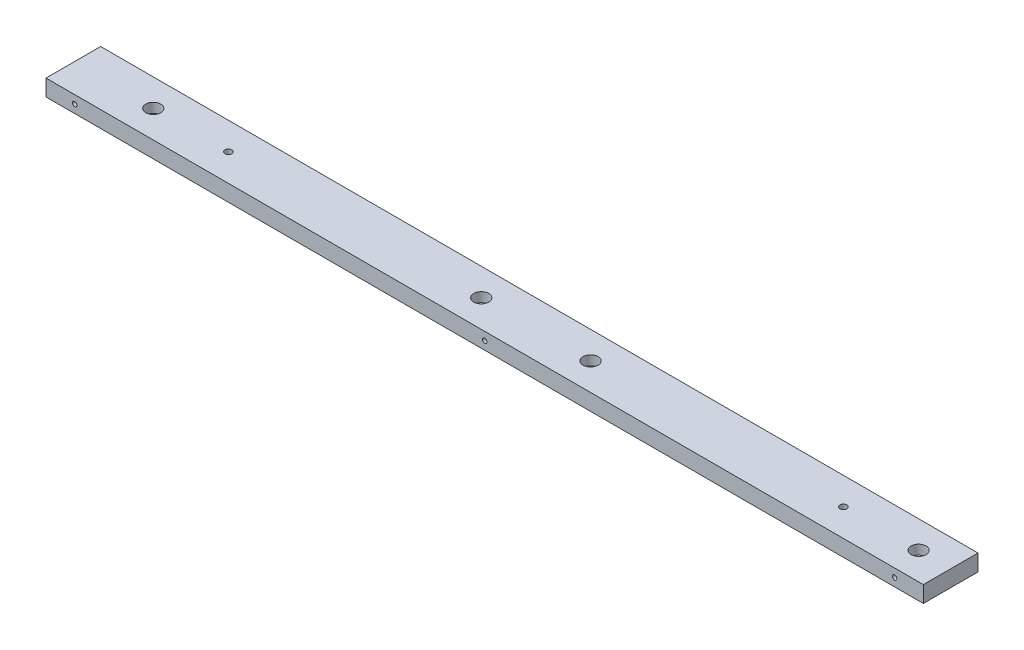
SolidWorks part; units mm, degrees
material "45#"
ref_plane "Front Plane" through (0, 0, 0) normal (0, 0, 1) x (1, 0, 0)
ref_plane "Top Plane" through (0, 0, 0) normal (0, 1, 0) x (1, 0, 0)
ref_plane "Right Plane" through (0, 0, 0) normal (1, 0, 0) x (0, 0, -1)
sketch "Sketch1" plane through (0, 0, 0) normal (0, 1, 0) x (1, 0, 0)
  line L0 (321, 20) -> (-321, -20) construction
  line L1 (-321, 20) -> (321, 20)
  line L2 (-321, 20) -> (-321, -20)
  line L3 (-321, -20) -> (321, -20)
  line L4 (321, 20) -> (321, -20)
  dimension "D1" = 642
  dimension "D2" = 40
extrude "Extrude1" add sketch "Sketch1" along normal mid plane 12
sketch "Sketch3" plane through (0, 6, 0) normal (0, 1, 0) x (1, 0, 0)
  point P0 (-262.5, 0)
  point P1 (297.5, 0)
  point P2 (57.5, 0)
  point P4 (-22.5, 0)
hole_wizard "M6 Socket Head Cap Screw Counterbore1" positions "3D Sketch1" profile "Sketch4" counterbore size "M6" standard "ISO" end condition through all
sketch3d "3D Sketch1"
  point P0 (-262.5, 6, 0)
  point P3 (-22.5, 6, 0)
  point P6 (57.5, 6, 0)
  point P9 (297.5, 6, 0)
sketch "Sketch4" plane through (-262.5, 6, 0) normal (1, 0, 0) x (0, 0, 1)
  line L0 (0, 0) -> (0, 12)
  line L1 (0, 12) -> (3.3, 12)
  line L3 (3.3, 12) -> (3.3, 7)
  line L4 (3.3, 7) -> (5.5, 7)
  line L5 (5.5, 7) -> (5.5, 0)
  line L7 (5.5, 0) -> (0, 0)
  line L11 (0, -6.35) -> (0, 107.95) construction
  dimension "貫穿孔直徑" = 6.6
  dimension "貫穿孔深度" = 12
  dimension "柱孔直徑" = 11
  dimension "柱孔深度" = 7
sketch "Sketch5" plane through (0, 0, 20) normal (0, 0, 1) x (1, 0, 0)
  point P0 (-300, 0)
  point P3 (0, 0)
  point P7 (300, 0)
hole_wizard "M4 Tapped Hole1" positions "3D Sketch2" profile "Sketch6" tap size "M4" standard "ISO"
sketch3d "3D Sketch2"
  point P0 (300, 0, 20)
  point P6 (0, 0, 20)
  point P12 (-300, 0, 20)
sketch "Sketch6" plane through (300, 0, 20) normal (1, 0, 0) x (0, -1, 0)
  line L0 (0, 0) -> (0, 11.0914)
  line L1 (0, 11.0914) -> (1.65, 10.1)
  line L2 (1.65, 10.1) -> (1.65, 0)
  line L5 (1.65, 0) -> (0, 0)
  line L10 (0, 11.0914) -> (-1.65, 10.1) construction
  line L11 (0, -6.35) -> (0, 107.95) construction
  dimension "螺孔鑽直徑" = 3.3
  dimension "螺孔鑽深度" = 10.1
  dimension "導頭角度" = 118
cosmetic thread "Cosmetic Thread1" parameters "D1"=8, "D2"=4
cosmetic thread "Cosmetic Thread2" parameters "D1"=8, "D2"=4
cosmetic thread "Cosmetic Thread3" parameters "D1"=8, "D2"=4
sketch "Sketch7" plane through (0, 6, 0) normal (0, 1, 0) x (1, 0, 0)
  point P0 (242.5, 0)
  point P1 (-207.5, 0)
hole_wizard "M6 Tapped Hole1" positions "3D Sketch3" profile "Sketch8" tap size "M6" standard "ISO" end condition through all
sketch3d "3D Sketch3"
  point P0 (-207.5, 6, 0)
  point P3 (242.5, 6, 0)
sketch "Sketch8" plane through (-207.5, 6, 0) normal (1, 0, 0) x (0, 0, 1)
  line L0 (0, 0) -> (0, 12)
  line L1 (0, 12) -> (2.5, 12)
  line L2 (2.5, 12) -> (2.5, 0)
  line L5 (2.5, 0) -> (0, 0)
  line L11 (0, -6.35) -> (0, 107.95) construction
  dimension "貫穿螺孔鑽直徑" = 5
  dimension "貫穿螺孔鑽深度" = 12
cosmetic thread "Cosmetic Thread4" parameters "D2"=15
cosmetic thread "Cosmetic Thread5" parameters "D2"=15
